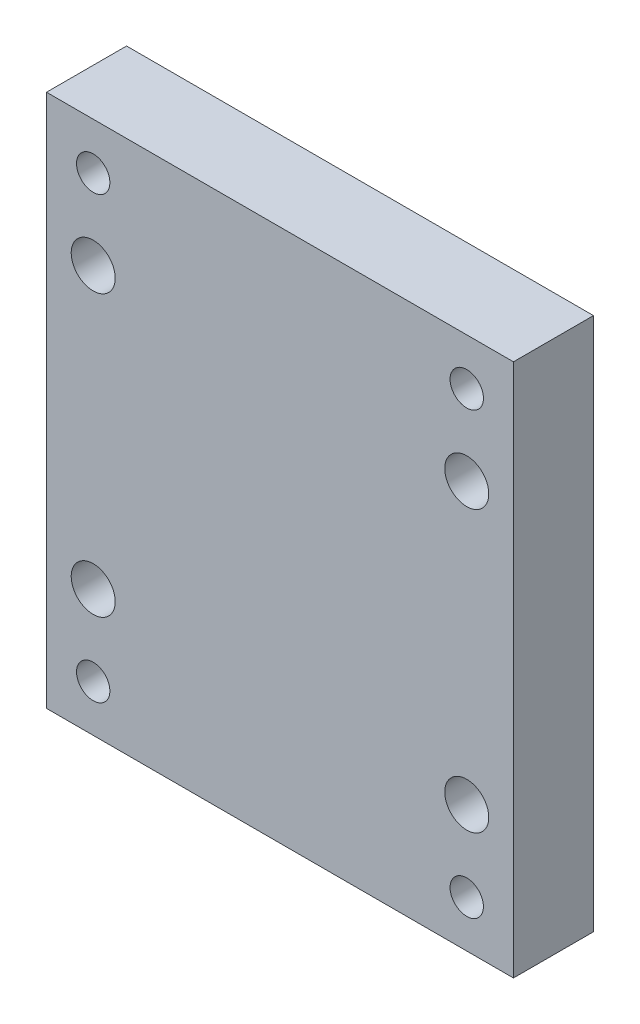
from build123d import *

# Parameters (mm, degrees)
SKETCH_1_W                     = 70
SKETCH_1_H                     = 80
EXTRUDE_1_DEPTH                = 12
HOLE_WIZARD_M6_1_D             = 5
HOLE_WIZARD_M6_1_2_D           = 6.6
HOLE_WIZARD_M6_1_2_CBORE_D     = 11
HOLE_WIZARD_M6_1_2_CBORE_DEPTH = 6.4


with BuildPart() as part:
    # 草图1 → 凸台-拉伸1 (new body)
    with BuildSketch(Plane.XY):
        Rectangle(SKETCH_1_W, SKETCH_1_H)
    extrude(amount=EXTRUDE_1_DEPTH)

    # Hole Wizard M6 _1 (through all)
    with Locations(Plane(origin=(0, 0, 0), x_dir=(-1, 0, 0), z_dir=(0, 0, -1))):
        with Locations((28, 33), (28, -33), (-28, -33), (-28, 33)):
            Hole(HOLE_WIZARD_M6_1_D / 2)

    # Hole Wizard M6 _1 2 (through all)
    with Locations(Plane(origin=(0, 0, 0), x_dir=(-1, 0, 0), z_dir=(0, 0, -1))):
        with Locations((-28, -21), (-28, 21), (28, -21), (28, 21)):
            CounterBoreHole(HOLE_WIZARD_M6_1_2_D / 2, HOLE_WIZARD_M6_1_2_CBORE_D / 2, HOLE_WIZARD_M6_1_2_CBORE_DEPTH)


solid = part.part
